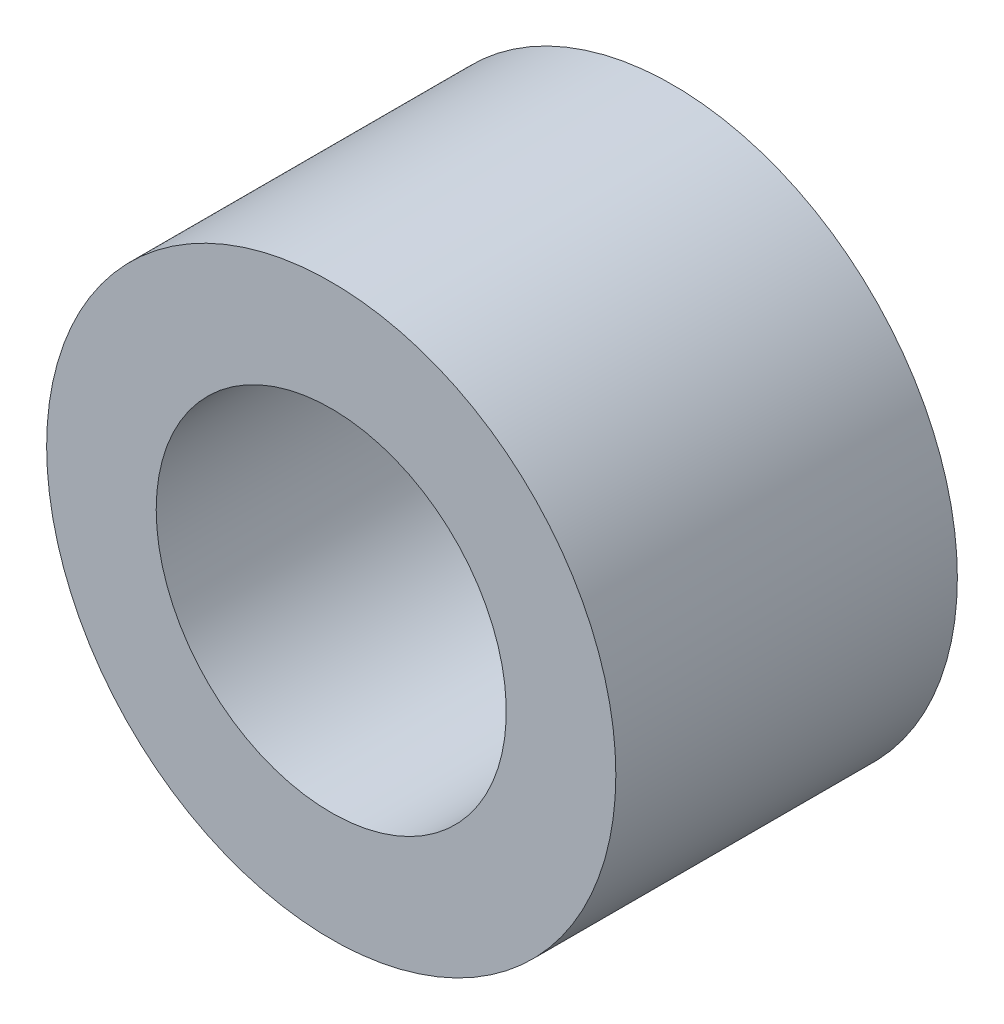
SolidWorks part; units mm, degrees
material "Q235"
ref_plane "Front Plane" through (0, 0, 0) normal (0, 0, 1) x (1, 0, 0)
ref_plane "Top Plane" through (0, 0, 0) normal (0, 1, 0) x (1, 0, 0)
ref_plane "Right Plane" through (0, 0, 0) normal (1, 0, 0) x (0, 0, -1)
sketch "Sketch1" plane through (0, 0, 0) normal (0, 0, 1) x (1, 0, 0)
  circle A0 centre (0, 0) radius 25
  dimension "D1" = 50
extrude "Boss-Extrude1" add sketch "Sketch1" along normal blind 30
hole_wizard "G1 Threaded hole1" positions "3DSketch1" profile "Sketch2" tap size "G1" standard "GB" end condition through all
sketch3d "3DSketch1"
  line L0 (0, 0, 30) -> (0, 0, 0) construction
  point P0 (0, 0, 0)
  point P3 (0, 0, 0)
  point P7 (0, 0, 0)
sketch "Sketch2" plane through (0, 0, 0) normal (1, 0, 0) x (0, 1, 0)
  line L0 (0, 0) -> (0, 30)
  line L1 (0, 30) -> (15.375, 30)
  line L2 (15.375, 30) -> (15.375, 0)
  line L5 (15.375, 0) -> (0, 0)
  line L11 (0, -6.35) -> (0, 107.95) construction
  dimension "通孔螺纹孔钻头直径" = 30.75
  dimension "通孔螺纹孔钻头深度" = 30
cosmetic thread "孔螺蚊线1" parameters "D2"=33.249
cosmetic thread "孔螺蚊线2" parameters "D2"=33.249
cosmetic thread "孔螺蚊线3" parameters "D2"=33.249
